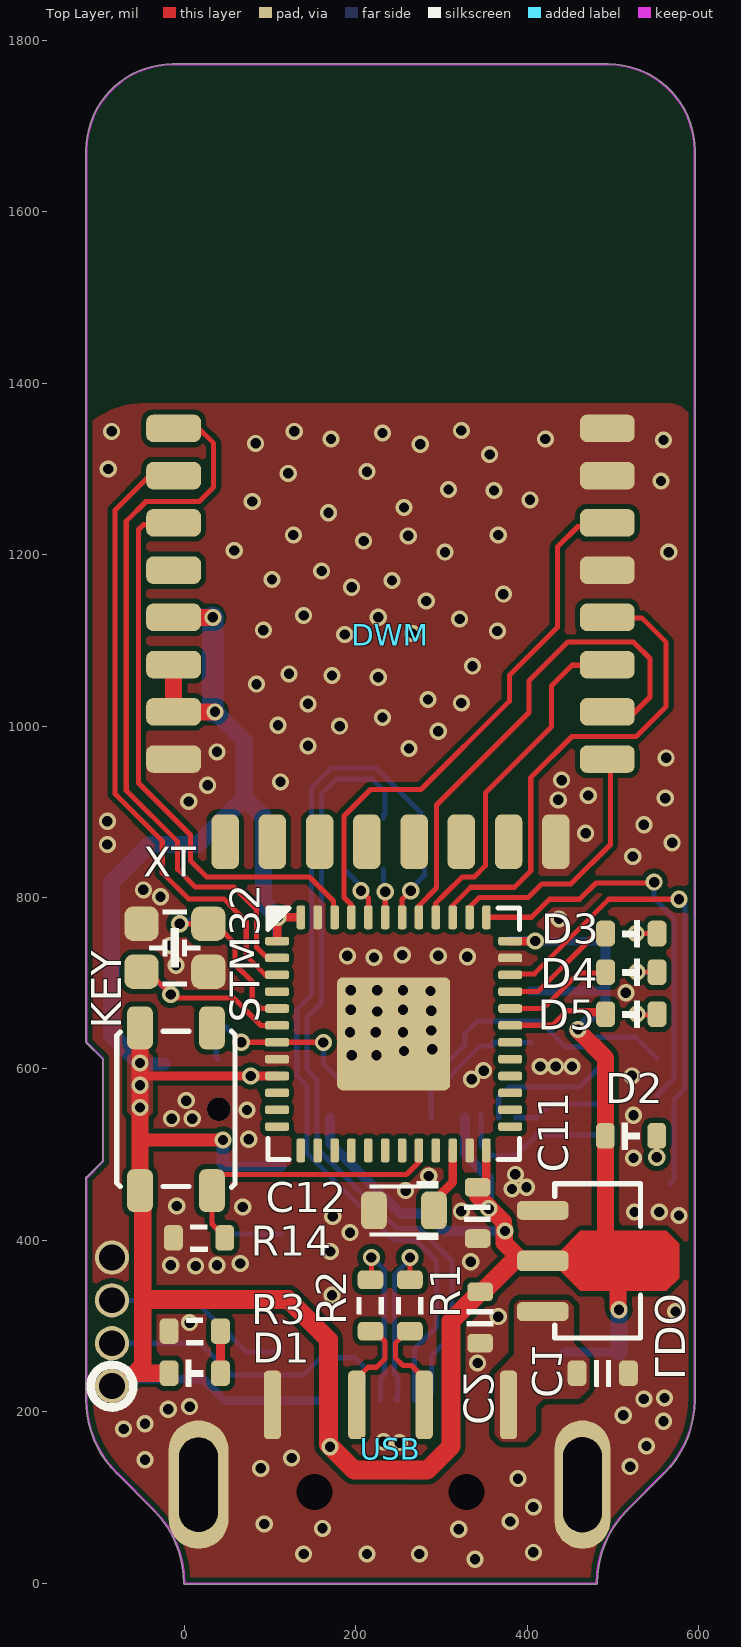
[diagram p0: Top Layer view]
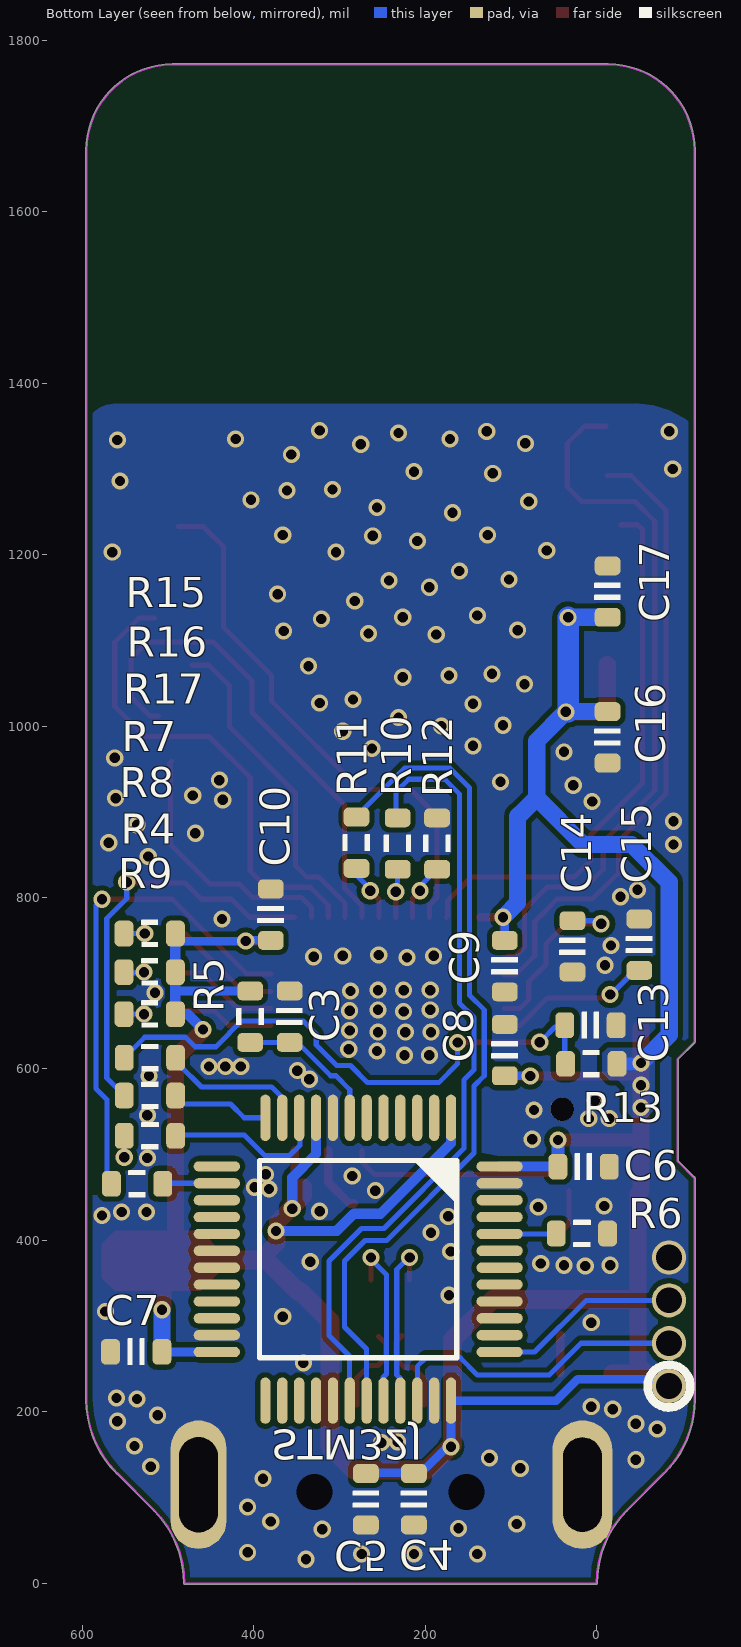
[diagram p1: Bottom Layer view, seen from below]
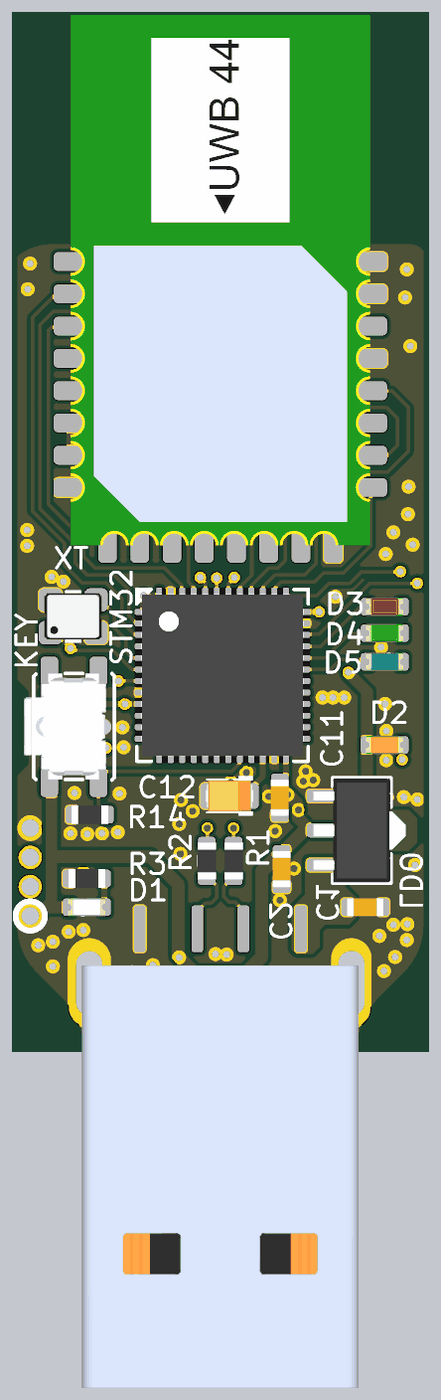
[diagram p2: 3D render of the assembled board from above, using the file's embedded part models]
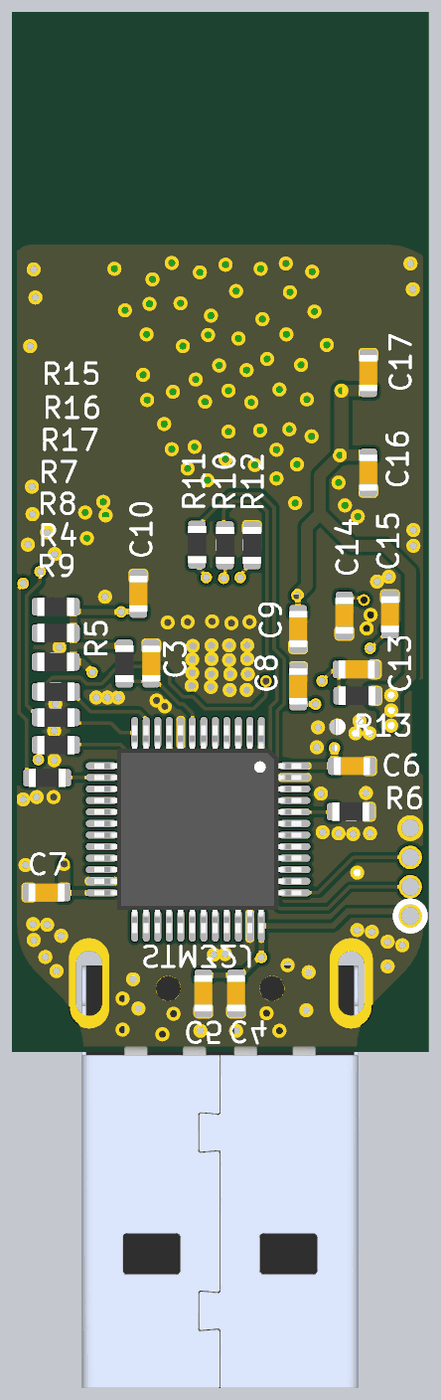
[diagram p3: 3D render of the assembled board from below, using the file's embedded part models]
# Altium PCB MISC82313-9.PcbDoc
Units mil, origin at the board's own origin, x right, y up, seen from the top; angles counter-clockwise.
Board outline 710.69 x 1773.68 mil, 2 copper layers (Top Layer, Bottom Layer), stack 49.606 mil thick; 46 components, 63 nets, 223 pads, 188 vias.

## Layer stack, top to bottom
Top Layer: signal copper 1.1811
Dielectric: core 47.2441, Dk 4.2
Bottom Layer: signal copper 1.1811

## Board outline
-115.01,214.02 -115.01,473 cw(c-114,473) -114.09,474.01 -95.68,492.42 -95.68,611.58 -114.71,630.61 cw(c-114,631.33) -114.72,630.62 -114.72,630.61 cw(c-114,631.33) -115.01,631.33 -115.01,1671.65 cw(c-14,1671.65) -14,1772.67 494.66,1772.67 cw(c494.66,1671.65) 595.68,1671.65 595.68,214.02 cw(c473.95,214.02) 560.02,127.94 516.72,84.64 ccw(c601.36,0) 481.66,0 cw(c480.65,0) 480.65,-1.01 0.02,-1.01 cw(c0.02,0) -1,0 ccw(c-120.69,0) -36.06,84.64 -79.36,127.94 ccw(c-78.64,128.66) -79.35,127.93 -79.36,127.94 cw(c6.71,214.02)

## Design rules (kind name [scope] priority, off if disabled: settings)
Clearance [All] p1: gap=6
ComponentClearance [All] p1: gap=0 collisioncheckmode=3 verticalgap=0 showdistances=FALSE
Height [All] p1: minheight=0 maxheight=5000 prefheight=500
HoleSize [All] p1: absolutevalues=TRUE maxlimit=200 minlimit=1 maxpercent=80.000 minpercent=20.000
HoleToHoleClearance [All] p1: gap=0 allowstackedmicrovias=TRUE
MinimumSolderMaskSliver [All] p1: minsoldermaskwidth=0
PolygonConnect [All] p1: connectstyle=Direct reliefconductorwidth=10 reliefentries=4 polygonreliefangle="90 Angle"
RoutingVias [All] p1: holewidth=12 width=20 viastyle="Through Hole" minholewidth=12 minwidth=20 maxholewidth=12 maxwidth=20
SilkToSilkClearance [All] p1: silktosilkclearance=0
SilkscreenOverComponentPads SilkToSolderMaskClearance [IsPad] p1: minsilkscreentomaskgap=0
SolderMaskExpansion [All] p1: expansion=2
Width [All] p1: maxlimit=50 minlimit=6 preferedwidth=10
21 further rules are at their usual default settings.

## Components (designator, comment, footprint, x,y, rotation, side; value= is the part's Value field where it differs from the comment)
C1 "Cap_0603" CAP_0603 488,245 r180 top
C2 "Cap_0603" CAP_0603 345,310 r90 top
C3 "Cap_0603" CAP_0603 358,661 r270 bottom
C4 "Cap_0603" CAP_0603 213,98 r90 bottom
C5 "Cap_0603" CAP_0603 269,98 r90 bottom
C6 "Cap_0603" CAP_0603 15,486 r0 bottom
C7 "Cap_0603" CAP_0603 537,270 r180 bottom
C8 "Cap_0603" CAP_0603 107,622 r270 bottom
C9 "Cap_0603" CAP_0603 107,720 r90 bottom
C10 "Cap_0603" CAP_0603 380,780 r270 bottom
C11 "Cap_0603" CAP_0603 342,432 r90 top
C12 "Cap_Tan_0805" CAP_TAN_P0805 256,435 r180 top
C13 "Cap_0603" CAP_0603 7,651 r0 bottom
C14 "Cap_0603" CAP_0603 28,743 r90 bottom
C15 "Cap_0603" CAP_0603 -50,745 r270 bottom
C16 "Cap_0603" CAP_0603 -13,987 r270 bottom
C17 "Cap_0603" CAP_0603 -13,1157 r90 bottom
D1 "LED_0603" LED_0603_YELLOW 12,245 r0 top
D2 "LED_0603" LED_0603_ORANGE 521,522 r0 top
D3 "LED_0603" LED_0603_RED 521.33,758 r180 top
D4 "LED_0603" LED_0603_GREEN 521.33,713 r180 top
D5 "LED_0603" LED_0603_BLUE 521.33,664 r180 top
DWM "DWM1000" DWM1000 240.33,863.15 r0 top locked
KEY "ButtonTACT" ButtonTACT_3.5*3.55_90 -10,553 r90 top
LDO "AMS1117" SOT89-3 482,376 r0 top
R1 "Res_0603" RES_0603 263,324 r90 top
R2 "Res_0603" RES_0603 217,324 r90 top
R3 "Res_0603" RES_0603 12,294 r0 top
R4 "Res_0603" RES_0603 521,522 r0 bottom
R5 "Res_0603" RES_0603 404,661 r90 bottom
R6 "Res_0603" RES_0603 17,408 r0 bottom
R7 "Res_0603" RES_0603 521,613 r180 bottom
R8 "Res_0603" RES_0603 521,569 r180 bottom
R9 "Res_0603" RES_0603 536,466 r180 bottom
R10 "Res_0603" RES_0603 232,863 r90 bottom
R11 "Res_0603" RES_0603 280,864 r90 bottom
R12 "Res_0603" RES_0603 186,863 r90 bottom
R13 "Res_0603" RES_0603 6,606 r180 bottom
R14 "Res_0603" RES_0603 17,403 r0 top
R15 "Res_0603" RES_0603 521.33,758 r180 bottom
R16 "Res_0603" RES_0603 521.33,713 r180 bottom
R17 "Res_0603" RES_0603 521.33,664 r180 bottom
STM32 "STM32F411C" QFN_P0.5_48 244,641 r0 top
STM32J "STM32F072C" LQFP_P0.5_48 278,378 r270 bottom
USB "USB_Plug_TypeA" USB_Plug_TypeA 240.33,0 r270 top
XT "XTAL_2520_4P" XT_2520_4 -11.17,741.5 r0 top

## Footprints (in the part's own frame and the unit in brackets; to place one, negate y for a bottom-side part, rotate by r counter-clockwise, add the part's x,y. Pads: shape width x height; smd on the part's side, far side on the other; paste and mask are expansions set on the pad)
ButtonTACT_3.5*3.55_90 [mil]
  round 27.56 hole 27.56 mask+0: 0(-0.01,-50)
  rrect50% 50x30 smd: 1(-95,42) 2(-95,-42) 3(95,42) 4(95,-42)
  silkscreen extent -91,-69 91,69, body extent -90,-55 91,85, height 56
CAP_0603 [mil]
  rrect50% 22x30 smd: 1(-30,0) 2(30,0)
  silkscreen extent -10,-15 10,15, body extent -31,-16 31,16, height 31
CAP_TAN_P0805 [mil]
  rrect50% 30x44 smd: 1(-35,0) 2(35,0)
  silkscreen extent -40,-34 40,34, body extent -40,-27 40,27, height 59
DWM1000 [mil]
  rrect50% 64x32 smd: 1(-253,484.25) 2(-253,429.13) 3(-253,374.02) 4(-253,318.9) 5(-253,263.78) 6(-253,208.66) 7(-253,153.54) 8(-253,98.43) 17(253,98.43) 18(253,153.54) 19(253,208.66) 20(253,263.78) 21(253,318.9) 22(253,374.02) 23(253,429.13) 24(253,484.25)
  rrect50% 32x64 smd: 9(-192.91,2) 10(-137.8,2) 11(-82.68,2) 12(-27.56,2) 13(27.56,2) 14(82.68,2) 15(137.8,2) 16(192.91,2)
  body extent -256,0 256,906, height 114
LED_0603_BLUE [mil]
  rrect50% 22x30 smd: 1(-30,0) 2(30,0)
  silkscreen extent -10,-16 10,16, body extent -32,-16 32,16, height 24
LED_0603_GREEN [mil]
  rrect50% 22x30 smd: 1(-30,0) 2(30,0)
  silkscreen extent -10,-16 10,16, body extent -32,-16 32,16, height 24
LED_0603_ORANGE [mil]
  rrect50% 22x30 smd: 1(-30,0) 2(30,0)
  silkscreen extent -10,-16 10,16, body extent -32,-16 32,16, height 24
LED_0603_RED [mil]
  rrect50% 22x30 smd: 1(-30,0) 2(30,0)
  silkscreen extent -10,-16 10,16, body extent -32,-16 32,16, height 24
LED_0603_YELLOW [mil]
  rrect50% 22x30 smd: 1(-30,0) 2(30,0)
  silkscreen extent -10,-16 10,16, body extent -32,-16 32,16, height 24
LQFP_P0.5_48 [mil]
  oval 54x12 smd: 1(-165,108.27) 2(-165,88.58) 3(-165,68.9) 4(-165,49.21) 5(-165,29.53) 6(-165,9.84) 7(-165,-9.84) 8(-165,-29.53) 9(-165,-49.21) 10(-165,-68.9) 11(-165,-88.58) 12(-165,-108.27) 25(165,-108.27) 26(165,-88.58) 27(165,-68.9) 28(165,-49.21) 29(165,-29.53) 30(165,-9.84) 31(165,9.84) 32(165,29.53) 33(165,49.21) 34(165,68.9) 35(165,88.58) 36(165,108.27)
  oval 12x54 smd: 13(-108.27,-165) 14(-88.58,-165) 15(-68.9,-165) 16(-49.21,-165) 17(-29.53,-165) 18(-9.84,-165) 19(9.84,-165) 20(29.53,-165) 21(49.21,-165) 22(68.9,-165) 23(88.58,-165) 24(108.27,-165) 37(108.27,165) 38(88.58,165) 39(68.9,165) 40(49.21,165) 41(29.53,165) 42(9.84,165) 43(-9.84,165) 44(-29.53,165) 45(-49.21,165) 46(-68.9,165) 47(-88.58,165) 48(-108.27,165)
  silkscreen extent -115,-115 115,115, body extent -177,-178 177,177, height 61
QFN_P0.5_48 [mil]
  rrect50% 28x10 smd: 1(-136,108.27) 2(-136,88.58) 3(-136,68.9) 4(-136,49.21) 5(-136,29.53) 6(-136,9.84) 7(-136,-9.84) 8(-136,-29.53) 9(-136,-49.21) 10(-136,-68.9) 11(-136,-88.58) 12(-136,-108.27) 25(136,-108.27) 26(136,-88.58) 27(136,-68.9) 28(136,-49.21) 29(136,-29.53) 30(136,-9.84) 31(136,9.84) 32(136,29.53) 33(136,49.21) 34(136,68.9) 35(136,88.58) 36(136,108.27)
  rrect50% 10x28 smd: 13(-108.27,-136) 14(-88.58,-136) 15(-68.9,-136) 16(-49.21,-136) 17(-29.53,-136) 18(-9.84,-136) 19(9.84,-136) 20(29.53,-136) 21(49.21,-136) 22(68.9,-136) 23(88.58,-136) 24(108.27,-136) 37(108.27,136) 38(88.58,136) 39(68.9,136) 40(49.21,136) 41(29.53,136) 42(9.84,136) 43(-9.84,136) 44(-29.53,136) 45(-49.21,136) 46(-68.9,136) 47(-88.58,136) 48(-108.27,136)
  rrect10% 132x132 smd: 49(0,0)
  silkscreen extent -147,-147 147,147, body extent -139,-139 139,139, height 22
RES_0603 [mil]
  rrect50% 22x30 smd: 1(-30,0) 2(30,0)
  silkscreen extent -10,-16 10,16, body extent -31,-16 31,16, height 18
SOT89-3 [mil]
  rrect50% 60x22 smd: 1(-64,59.06) 3(-64,-59.06)
  rrect50% 60x24 smd: 2(-64,0)
  Top Layer region: -45,10 -20,35 80,35 95,20 95,-20 80,-35 -20,-35 -45,-10
  silkscreen extent -50,-90 50,90, body extent -83,-88 75,88, height 60
USB_Plug_TypeA [mil]
  round 32 hole 42: 0(-106.3,88.58) 0(-106.3,-88.58)
  rrect50% 80x20 smd: 1(-208,137.8) 2(-208,39.37) 3(-208,-39.37) 4(-208,-137.8)
  oval 150x65 hole 45 slot 111 at 0 deg: 4(-115,224)
  oval 150x70 hole 45 slot 110 at 0 deg: 4(-115,-224)
  body extent -146,-236 576,236, height 70
XT_2520_4 [mil]
  rrect50% 40x40 smd: 1(39,28) 2(-39,28) 3(-39,-28) 4(39,-28)
  silkscreen extent -30,-44 30,44, body extent -49,-39 49,39, height 31

## Part data
C1 C2 C3 C4 C5 C6 C7 C8 C9 C10 C11 C12 C13 C14 C15 C16 C17: "Capacitor"
D1 D2 D3 D4 D5: "LED"
DWM: "Module"
KEY: "Button"
LDO: library part LDO1117, "Power"
R1 R2 R3 R4 R5 R6 R7 R8 R9 R10 R11 R12 R13 R14 R15 R16 R17: "Resistor"
STM32: library part STM32F4x1C, "MCU"
STM32J: library part STM32F103C, "MCU"
USB: "USB"
XT: "Crystal Oscillator"

## Free pads (board coordinates)
  round 40 hole 30: 1(-84.67,230) 2(-84.67,280) 3(-84.67,330) 4(-84.67,380)

## Via types
v1: diameter 20, hole 12, Top Layer to Bottom Layer, 188 vias

## Nets (pads, with @x,y where several pads share a name; then routed paths per layer and width w, separated by ;. In a path a pad name is that pad's centre, name@x,y a point inside that pad or via, vN(x,y) a via of type N, cw(c..) or ccw(c..) an arc to the next point about the centre after c; other vN are vias at no path point)
3V3: C2.2 C4.2 C5.2 C6.2 C7.2 C8.2 C9.2 C10.2 C11.2 C16.1 C17.1 D1.1 D2.1 DWM.5 DWM.6 DWM.7 KEY.1 KEY.3 LDO.2 pad.1 R5.2 R13.2 R15.2 R16.2 R17.2 STM32.1 STM32.9 STM32.24 STM32.36 STM32.48 STM32J.1 STM32J.9 STM32J.24 STM32J.36 STM32J.48 | length 4548.4
  Top Layer w10: -49.79,591.79 v1(77.21,591.79) STM32.9 ; STM32.1 v1@108,770 ; v1(109,777) STM32.48 ; C11.2@349,466 352.27,469.27 STM32.24 ; STM32.36 v1(409.27,749.27) ; D2.1@491,516 D2.1
  Top Layer w15: pad.1 pad.1@-73.33,241.33 ; pad.1@-69,237 pad.1@-67.5,238.5 ; -48,517 v1(45,517)
  Top Layer w20: pad.1@-66,237 -48.67,254.33 -48.67,454.67 KEY.1 ; -57,245 D1.1 ; KEY.1@-52,463 KEY.3 ; DWM.7 v1(35.69,1016.69) ; DWM.6 -12.67,1021.67 DWM.7@-11,1020 ; DWM.5 v1(33.07,1126.93) ; C11.2 342,452 372,422 v1@372,420.49 ; v1@373,414 373,397 LDO.2@393,377 ; v1@459,645 491,613 D2.1 491,400 492,399 ; 489,377 489,399 ; 505,354 506,353 v1@506,322
  Top Layer w22: -46,331 121,331 168,284 v1@168,162 ; v1@170.23,159.77 198,132 283,132 311,160 311,306 C2.2 ; C2.2@348,340 385,377 393,377 453,377
  Bottom Layer w10: pad.1@-73,238 22,238 47,213 STM32J.36 v1@169.73,163.27 ; v1@78,592 C8.2 ; C9.2 v1@107,773 ; v1@171.73,161.27 204,129 266,129 C5.2@270,125 ; C10.2 v1@404,750 ; R5.2 489,691 490,692 ; v1(409.27,749.27) R15.2@490.73,749.27 ; STM32J.24 C7.2@508.73,269.73
  Bottom Layer w12: C6.2@45.27,486.27 STM32J.48 ; STM32J.1 169.73,513.27 252,431 283,431 303,411 v1(374,411) ; STM32J.9 327.21,500.79 355,473 v1(355,437) ; v1(459,646) 477,664 R17.2@491,664 ; R17.2 R17.2@491,664 ; R15.2 R16.2 491.33,664.33 R17.2@491,664
  Bottom Layer w15: v1@-50,606 R13.2 ; C6.2@45,490 v1(45,517)
  Bottom Layer w20: v1(-52,607) -85,640 -85,818 -41,862 15.39,862 69.69,916.31 ; C16.1 v1@32,1017 ; C17.1 v1@28,1127 ; v1(35.69,1016.69) 69.69,982.69 69.69,916.31 ; 90,896 ccw(c89.5,896) 89.5,896.5 ; v1@108,778 92,794 92,894 ccw(c89.5,894) 89.5,896.5 ; C7.2 v1(507,319) ; 69.69,916.31 89.5,896.5
  Bottom Layer w25: v1@33.07,1016.93 v1(33.07,1126.93)
  other v1: 169.73,159.27 -52,555 -52,581
BOOT: R12.1 STM32.44 | length 65.2
  Top Layer w6: v1(206,808) 214.47,799.53 STM32.44
  Bottom Layer w6: R12.1 207,812 v1@207,811
D_CS: DWM.17 STM32.38 | length 304.2
  Top Layer w6: STM32.38 332.58,788.58 344,800 401,800 417,816 451,816 497,862 DWM.17@497,954 ; DWM.17@496,959 498,957 DWM.17@498,954
D_EXT: DWM.1 STM32.2 | length 837.7
  Top Layer w6: DWM.1@-11,1350 14,1350 34,1330 34,1279 17.17,1262.17 -44.83,1262.17 -68,1239 -68,925 -8,865 -8,833 12.85,812.15 57.85,812.15 84,786 84,742 95,731 STM32.2@104,731 ; STM32.2@104,729.58 STM32.2
D_IRQ: DWM.22 STM32.45 | length 636.3
  Top Layer w6: STM32.45 194.79,791.21 186,800 186,895 217,926 276,926 379,1029 379,1059 435,1115 435,1209 459,1233 DWM.22@488,1233
D_PHA: DWM.9
D_POL: DWM.10
D_RST: DWM.3 STM32.46 | length 644.4
  Top Layer w6: DWM.3@-29,1235 -48,1235 -53.67,1229.33 -53.67,933.67 7,873 7,843 25.85,824.15 145.85,824.15 174,796 174,778.1 STM32.46
D_SCK: DWM.20 STM32.39 | length 555.6
  Top Layer w6: STM32.39 312.9,790.9 334,812 385,812 404,831 404,940 452,988 491,988 527,988 562,1023 562,1098 534,1126 DWM.20@516,1126
D_SDI: DWM.18 STM32.41 | length 582.8
  Top Layer w6: STM32.41 273.53,790.53 294,811 294,908 402,1016 402,1053 447,1098 524,1098 543,1079 543,1034 521,1012 DWM.18@511,1012
D_SDO: DWM.19 STM32.40 | length 388
  Top Layer w6: STM32.40 293.21,793.24 303.99,804.01 ; 304,804 324.15,824.15 338.15,824.15 351,837 351,922 428,999 428,1047 452,1071 DWM.19@472,1071
D_WAK: DWM.2 STM32.3 | length 737.7
  Top Layer w6: DWM.2 -40.72,1292.28 -81,1252 -81,921 -26,866 -26,829 4.5,798.5 45.7,798.5 56.83,787.37 56.83,787.17 58,786 59,785 72,772 72,732 94.1,709.9 STM32.3
GND: C1.1 C2.1 C3.1 C4.1 C5.1 C6.1 C7.1 C8.1 C9.1 C10.1 C11.1 C12.2 C13.1 C14.1 C15.1 C16.2 C17.2 DWM.8 DWM.16 DWM.21 DWM.23 DWM.24 KEY.0 LDO.1 pad.4 R3.1 R6.1 R12.2 R14.1 STM32.8 STM32.23 STM32.35 STM32.47 STM32.49 STM32J.8 STM32J.23 STM32J.35 STM32J.47 USB.0 USB.4 XT.2 XT.4
  other v1: 339,28 139,34 213,34 274,34 407,36 320,63 161,64 93,69 380,72 407,89 389,122 89,134 520,136 -46,144 125,146 539,160 251,164 232,165 -71,180 -46,186 559,189 512,196 -19,203 6,206 536,215 560,216 342,257 6,304 366,311 573,317 172,336 13,370 -16,371 38,371 65,373 334,375 170,387 193,409 173,428 577,429 525,433 554,433 323,434 68,439 -9,440 258,458 382,460 399,462 285,475 386,477 524,496 75,518 -15,542 9,542 524,546 73,552 2,563 335,588 522,592 349,598 415,603 433,603 452,603 195,616 224,616 256,621 289,623 193,643 223,643 255,643 288,645 225,667 288,668 194,669 255,669 515,689 287,691 194,692 225,692 255,692 -10,721 221,730 330,731 190,732 296,732 254,733 -17,744 437,775 -28,801 -48,809 523,848 -90,862 569,864 468,875 536,885 -90,889 5,912 436,914 561,916 471,919 27,931 112,935 440,937 562,963 38,970 262,974 144,977 296,994 181,1000 109,1001 231,1010 144,1026 323,1027 284,1031 84,1049 226,1057 172,1059 122,1061 336,1070 187,1107 266,1108 365,1111 92,1112 321,1125 226,1127 139,1129 282,1146 372,1154 195,1162 242,1170 102,1171 160,1181 304,1203 565,1203 58,1205 209,1216 261,1222 127,1223 366,1223 168,1249 256,1255 79,1262 403,1264 361,1275 308,1276 556,1286 121,1295 213,1297 -89,1300 356,1317 275,1329 83,1330 559,1334 171,1335 421,1335 231,1342 -85,1344 128,1344 323,1345
ISWCLK: pad.3 STM32J.37 | length 218
  Bottom Layer w6: pad.3@-80,330 12,330 72.27,269.73 STM32J.37
ISWDIO: pad.2 STM32J.34 | length 346.4
  Bottom Layer w6: pad.2 18,280 55,243 121,243 139,243 159,263 199,263 209,253 STM32J.34@209,228
JBOOT: R6.2 STM32J.44 | length 57.5
  Bottom Layer w6: R6.2@55.47,407.53 STM32J.44
JRST: C13.2 R7.1 R13.1 STM32.7 | length 662
  Top Layer w6: v1(66.16,631.16) STM32.7 v1@161.84,631.16
  Bottom Layer w6: R13.1@39,611 37,613 C13.2 C13.2@40,648 ; C13.2@41,649 48.31,649 v1@63.31,634 ; v1@66,631 v1(66.16,631.16) v1@63.31,634 ; v1@66,634 v1@63.31,634 ; v1@162,629 162,606 184,584 267,584 287,604 303,604 327,628 327,641 342,656 414,656 419,651 419.51,651 428,642.51 428,642 444,626 468.49,626 479.49,637 527,637 R7.1
  other v1: 162,631
JRX: R11.1 STM32.42 | length 63
  Top Layer w6: STM32.42 253.84,797.84 v1(264,808)
  Bottom Layer w6: v1@266,812 280,826 R11.1
JSC: R8.1 STM32.37 | length 496.6
  Top Layer w6: STM32.37 369,777 ; 372,777 369,777 ; v1@546,817 480,817 461,798 426,798 405,777 369,777 ; v1@546,818 v1(548,818) v1@553,818
  Bottom Layer w6: v1(548,818) 548,799 571.33,775.67 571.33,589.33 R8.1 ; R8.1@552,569 R8.1@558.5,575.5
JSD: R9.1 STM32.34 | length 574
  Top Layer w6: STM32.34@380,711 408,711 495,798 v1(577,798)
  Bottom Layer w6: R9.1 571,471 571,564 584,577 584,791 v1@578,797
JTX: R10.1 STM32.43 | length 54.3
  Top Layer w6: STM32.43 v1(234.16,806.84)
  Bottom Layer w6: R10.1 232,810 v1@233,809
KEY: KEY.2 R14.2 STM32.20 | length 310.8
  Top Layer w6: KEY.2 32,419 R14.2@45,406 ; KEY.2@40,476 41,477 259,477 273.53,491.53 STM32.20
LED: R4.1 STM32J.10 | length 194.9
  Bottom Layer w6: STM32J.10@346,547 346,511 358,499 387,499 411,523 R4.1@490,523
LED_B: D5.2 STM32.31 | length 128
  Top Layer w6: STM32.31 STM32.31@383,650.84 ; STM32.31@383,651 429,651 446,668 481,668 D5.2@485,664 ; 477,664 D5.2@485,664 ; D5.2 D5.2@485,664
LED_G: D4.2 STM32.32 | length 131.2
  Top Layer w6: STM32.32 418.53,670.53 460,712 D4.2@494,712
LED_R: D3.2 STM32.33 | length 144.4
  Top Layer w6: STM32.33@385,690.21 STM32.33 412.21,690.21 480,758 D3.2
NetD1_2: D1.2 R3.2 | length 44.4
  Top Layer w10: R3.2@41,289 42,288 D1.2
NetD2_2: D2.2 R4.2 | length 47
  Top Layer w6: v1(551,497) D2.2
  Bottom Layer w6: v1(551,497) R4.2@551,519
NetD3_1: D3.1 R15.1 | length 48.2
  Top Layer w6: v1(527,758) 548,758 D3.1@550,756
  Bottom Layer w6: v1(527,758) R15.1
NetD4_1: D4.1 R16.1 | length 48.7
  Top Layer w6: v1(528,713) D4.1
  Bottom Layer w6: v1(528,713) 529,712 R16.1@553,712
NetD5_1: D5.1 R17.1 | length 43.7
  Top Layer w6: v1(528,664) 529,663 D5.1@548,663
  Bottom Layer w6: v1(528,664) R17.1
NetR1_1: R1.1 USB.2 | length 103.1
  Top Layer w6: R1.1@254,288 246,280 246,263 255,254 265,254 279.7,239.3 USB.2
NetR2_1: R2.1 USB.3 | length 103.4
  Top Layer w6: USB.3 200.96,238.96 214,252 224,252 234,262 234,282 R2.1@227,289
NetR7_2: R7.2 STM32J.11 | length 159.7
  Bottom Layer w6: STM32J.11 STM32J.11@366.58,567 ; STM32J.11@367,567 379,579 461,579 R7.2@487,605
NetR8_2: R8.2 STM32J.12 | length 126.1
  Bottom Layer w6: STM32J.12 411,543 427,559 483,559 492,568 R8.2@492,578
NetR9_2: R9.2 STM32J.14 | length 55.6
  Bottom Layer w6: STM32J.14 R9.2@498.58,466.58
NetR10_2: R10.2 STM32J.30 | length 918.6
  Bottom Layer w6: R10.2 R10.2@232,897 ; R10.2@234,897 234,923 219,938 177,938 160,921 160,677 143,660 143,599 154.73,587.27 154.73,507.05 247.79,414 274,414 312,376 312,289 288,265 STM32J.30@288,222
NetR11_2: R11.2 STM32J.31 | length 974.1
  Bottom Layer w6: STM32J.31 268.16,273.16 294,299 294,376 270,400 244.82,400 142.73,502.08 142.73,580.27 131,592 131,669 148,686 148,928 171,951 224,951 R11.2@276,899
PA0: STM32.10
PA1: STM32.11
PA2: STM32.12
PA3: STM32.13
PA4: STM32.14
PA5: STM32.15
PA6: STM32.16
PA7: STM32.17
PA8: STM32.29
PA9: STM32.30
PB0: STM32.18
PB1: STM32.19
PB\10: STM32.21
PB\12: STM32.25
PB\13: STM32.26
PB\14: STM32.27
PB\15: STM32.28
PC15: STM32.4
RST: C3.2 R5.1 STM32J.7 | length 172.4
  Bottom Layer w6: STM32J.7 287.84,575.84 304,592 310,592 345,627 359,627 C3.2@361,629 ; C3.2@360,632 361,631 R5.1
USB_DM: R1.2 STM32J.32 | length 203.6
  Top Layer w6: R1.2 v1(263,380)
  Bottom Layer w6: STM32J.32@246,215.47 STM32J.32 STM32J.32@248.47,222 ; STM32J.32@249,222 249,240 245,244 245,360 v1@263,378
USB_DP: R2.2 STM32J.33 | length 196.3
  Top Layer w6: R2.2@218,354 v1(218,380)
  Bottom Layer w6: v1@222,377 233,366 233,243 228.79,238.79 STM32J.33
VCAP: C12.1 STM32.22 | length 77.3
  Top Layer w10: C12.1@283,443 288,443 312.9,467.9 STM32.22
VUSB: C1.2 LDO.3 USB.1
XT_I: C14.2 STM32.5 XT.1 | length 194.8
  Top Layer w6: v1(-5.5,769.5) XT.1 ; XT.1@42,763 59,746 59,722 79,702 79,681 89.47,670.53 STM32.5
  Bottom Layer w6: v1@-2,771 0,773 C14.2
XT_O: C15.2 STM32.6 XT.3 | length 224.6
  Top Layer w6: XT.3@-45,716 v1(-16,687) -12,683 57,683 89.16,650.84 STM32.6
  Bottom Layer w6: C15.2 -45,715 v1@-17,687
pads on no net: DWM.4 DWM.11 DWM.12 DWM.13 DWM.14 DWM.15 KEY.4 STM32J.2 STM32J.3 STM32J.4 STM32J.5 STM32J.6 STM32J.13 STM32J.15 STM32J.16 STM32J.17 STM32J.18 STM32J.19 STM32J.20 STM32J.21 STM32J.22 STM32J.25 STM32J.26 STM32J.27 STM32J.28 STM32J.29 STM32J.38 STM32J.39 STM32J.40 STM32J.41 STM32J.42 STM32J.43 STM32J.45 STM32J.46

## Polygon pours and split planes (outlines as drawn)
GND on Top Layer "Top Layer-No Net" (solid, remove dead copper): -187.68,1334.93 -187.68,150.35 ccw(c-87.68,150.35) -158.39,79.64 -77.68,-1.07 -41.97,-36.78 ccw(c28.74,33.93) 28.74,-66.07 146.32,-66.07 496.9,-66.07 ccw(c496.9,33.93) 567.61,-36.78 615.32,10.93 646.03,41.64 ccw(c575.32,112.35) 675.32,112.35 675.32,434.93 673.61,436.64 cw(c744.32,507.35) 644.32,507.35 644.32,1253.93 644.32,1267.51 ccw(c544.32,1267.51) 615.03,1338.22 585.32,1367.93 ccw(c563.59,1346.2) 563.59,1376.93 528.32,1376.93 -46.26,1376.93 ccw(c-46.26,1276.93) -116.97,1347.64 -148.68,1315.93 -160.69,1303.92 ccw(c-90.7,1233.93) -189.68,1233.93
3V3 on Top Layer "Top Layer-No Net" (solid, remove dead copper): -67,611 -67,550 -63,546 -59,542 -54,542 -44,542 -41,545 -37,549 -37,559 -37,615 -41,619 -43,621 -49,621 -60,621 -66,615 -67,614 -67,611
VUSB on Top Layer "Top Layer-No Net" (solid, remove dead copper): 362,225 362,199 362,173 366,169 370,165 381,165 398,165 403,170 410,177 410,196 410,206 414,210 419,215 435,215 460,215 468,223 472,227 472,243 472,262 464,270 454,280 454,307 454,323 450,327 447,330 436,330 390,330 386,326 385,325 385,320 385,267 369,251 362,244 362,225
GND on Bottom Layer "Top Layer-No Net" (solid, remove dead copper): -188,1334 -188,149.42 ccw(c-88,149.42) -158.71,78.71 -78,-2 -42.29,-37.71 ccw(c28.42,33) 28.42,-67 146,-67 496.58,-67 ccw(c496.58,33) 567.29,-37.71 615,10 645.71,40.71 ccw(c575,111.42) 675,111.42 675,434 673.29,435.71 cw(c744,506.42) 644,506.42 644,1253 644,1266.58 ccw(c544,1266.58) 614.71,1337.29 585,1367 ccw(c563.27,1345.27) 563.27,1376 528,1376 -46.58,1376 ccw(c-46.58,1276) -117.29,1346.71 -149,1315 -161.01,1302.99 ccw(c-91.02,1233) -190,1233
3V3 on Bottom Layer "Top Layer-No Net" (solid, remove dead copper): -68,599 -68,553 -63,548 -58,543 -47,543 -42,543 -35,550 -33,552 -33,564 -33,579 -27,585 -25,587 -20,587 -16,587 -11,592 -7,596 -7,611 -7,619 -10,622 -13,625 -20,625 -53,625 -63,615 -68,610 -68,599

## Keep-outs
Keep-Out Layer:
  lines w2: -114,472.67 -94.67,492 -94.67,612 -114,631.33 -114,632 -114,1671.65 cw(c-14,1671.65) -14,1771.65 494.66,1771.65 cw(c494.66,1671.65) 594.66,1671.65 594.66,214.02 cw(c473.95,214.02) 559.31,128.66 516,85.36 ccw(c601.36,0) 480.65,0 0.02,0 ccw(c-120.69,0) -35.34,85.36 -78.64,128.66 cw(c6.71,214.02) -114,214.02 -114,473

## Silkscreen, mask and mechanical layers (free items; w line width, h text height)
Top Overlay:
  circle w10: c-84.67,230 r25
Bottom Overlay:
  circle w10: c-84.67,230 r25